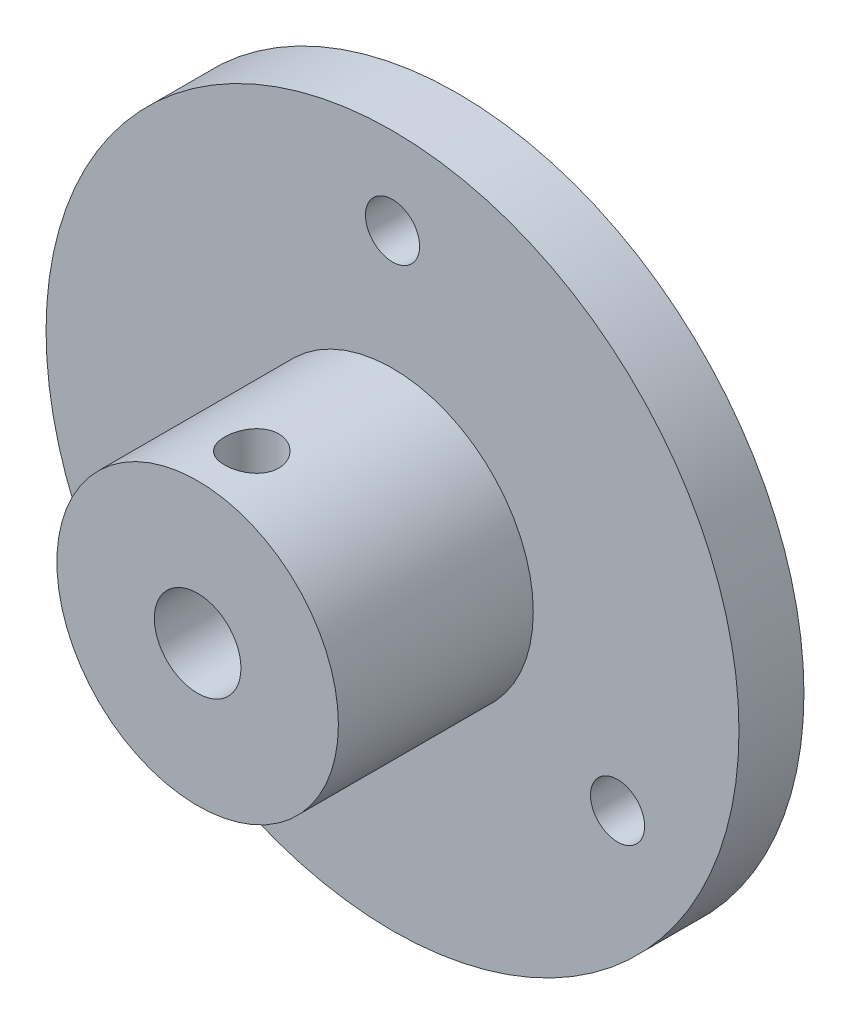
from build123d import *

# Parameters (mm, degrees)
SKETCH1_R             = 16
BOSS_EXTRUDE1_DEPTH   = 3
SKETCH2_R             = 6.5
BOSS_EXTRUDE2_DEPTH   = 9
SKETCH3_R             = 2
CUT_EXTRUDE1_DEPTH    = 22
SKETCH4_R             = 1
CUT_EXTRUDE2_DEPTH    = 10
M3_TAPPED_HOLE6_D     = 2.5
M3_TAPPED_HOLE6_DEPTH = 12


with BuildPart() as part:
    # Sketch1 → Boss-Extrude1 (new body)
    with BuildSketch(Plane.XY):
        Circle(SKETCH1_R)
    extrude(amount=BOSS_EXTRUDE1_DEPTH)

    # Sketch2 → Boss-Extrude2 (add)
    with BuildSketch(Plane.XY.offset(3)):
        Circle(SKETCH2_R)
    extrude(amount=BOSS_EXTRUDE2_DEPTH)

    # Sketch3 → Cut-Extrude1 (cut)
    with BuildSketch(Plane(origin=(0, 0, 0), x_dir=(-1, 0, 0), z_dir=(0, 0, -1))):
        Circle(SKETCH3_R)
    extrude(amount=-CUT_EXTRUDE1_DEPTH, mode=Mode.SUBTRACT)

    # Sketch16 → M3 Tapped Hole5 (revolve, cut)
    with BuildSketch(Plane(origin=(0, 0, 9.5), x_dir=(0, 0, -1), z_dir=(1, 0, 0))):
        Polygon((0, 0), (0, 8.251075774), (1.25, 7.5), (1.25, 0), align=None)
    revolve(axis=Axis((0, -6.35, 9.5), (0, 1, 0)), mode=Mode.SUBTRACT)

    # Sketch4 → Cut-Extrude2 (cut)
    with BuildSketch(Plane(origin=(0, 0, 0), x_dir=(-1, 0, 0), z_dir=(0, 0, -1))):
        with Locations((0, 12)):
            Circle(SKETCH4_R)
        with Locations((10.392304845, -6)):
            Circle(SKETCH4_R)
        with Locations((-10.392304845, -6)):
            Circle(SKETCH4_R)
    extrude(amount=-CUT_EXTRUDE2_DEPTH, mode=Mode.SUBTRACT)

    # M3 Tapped Hole6
    with Locations(Plane(origin=(0, 0, 0), x_dir=(-1, 0, 0), z_dir=(0, 0, -1))):
        with Locations((0, 12), (-10.392304845, -6), (10.392304845, -6)):
            Hole(M3_TAPPED_HOLE6_D / 2, depth=M3_TAPPED_HOLE6_DEPTH)


solid = part.part
